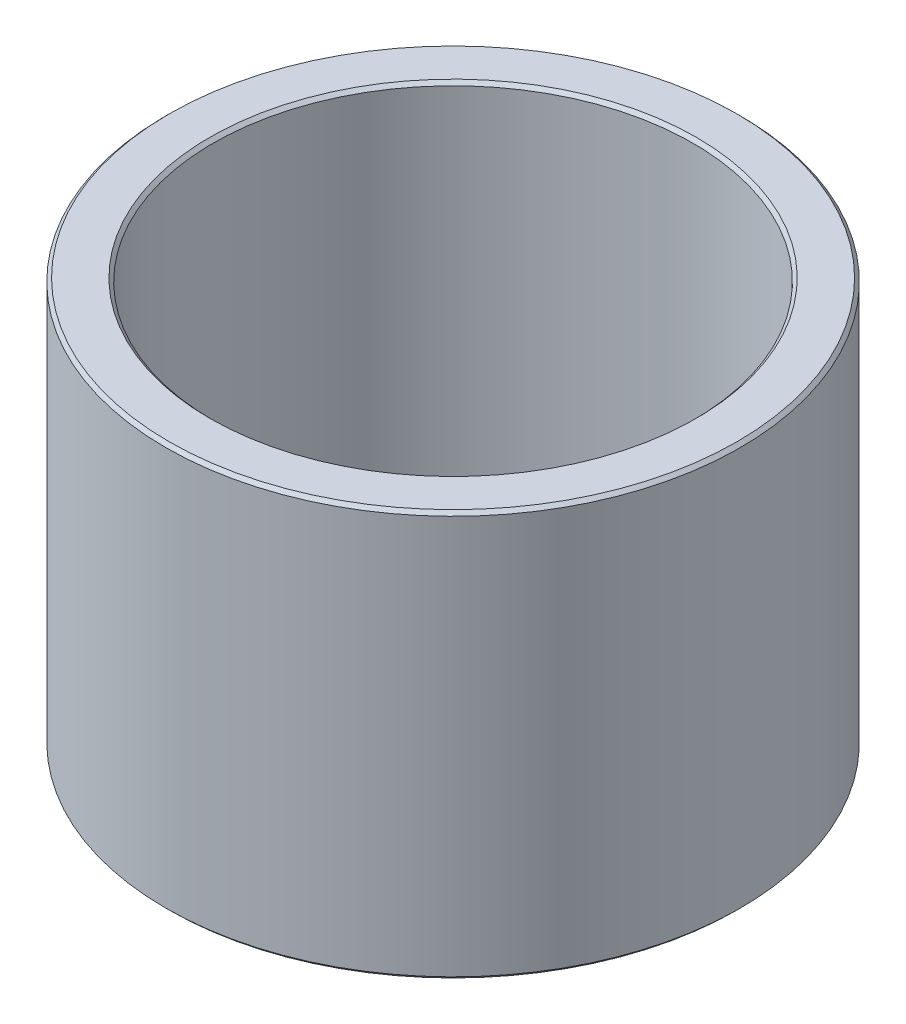
SolidWorks part; units mm, degrees
material "20 Steel"
ref_plane "Front Plane" through (0, 0, 0) normal (0, 0, 1) x (1, 0, 0)
ref_plane "Top Plane" through (0, 0, 0) normal (0, 1, 0) x (1, 0, 0)
ref_plane "Right Plane" through (0, 0, 0) normal (1, 0, 0) x (0, 0, -1)
other "Configuration Table"
sketch "Sketch1" plane through (0, 0, 0) normal (0, 1, 0) x (1, 0, 0)
  circle A0 centre (0, 0) radius 42.5
  circle A1 centre (0, 0) radius 35.5
  dimension "D1" = 71
  dimension "D2" = 85
extrude "Boss-Extrude1" add sketch "Sketch1" along normal blind 60
chamfer "Chamfer1" distance 0.5 angle 45 4 edges at (0, 60, 42.5) (0, 0, 42.5) (0, 60, 35.5) (0, 0, 35.5)
